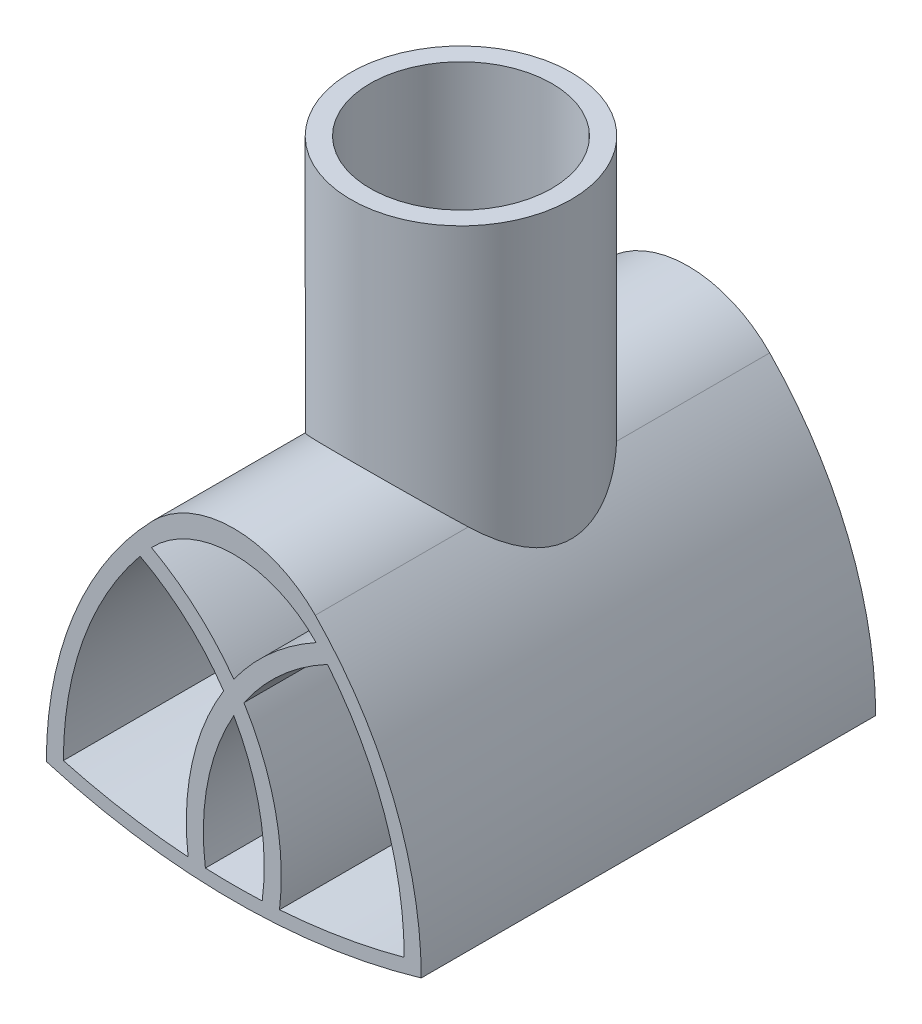
SolidWorks part; units mm, degrees
ref_plane "前视基准面" through (0, 0, 0) normal (0, 0, 1) x (1, 0, 0)
ref_plane "上视基准面" through (0, 0, 0) normal (0, 1, 0) x (1, 0, 0)
ref_plane "右视基准面" through (0, 0, 0) normal (1, 0, 0) x (0, 0, -1)
sketch "缓冲脚外形" plane through (0, 0, 0) normal (0, 0, 1) x (1, 0, 0)
  line L0 (0, 0) -> (0, -36980.811) construction
  line L1 (0, 0) -> (36980.811, 0) construction
  arc A0 (-15, 2) -> (15, 2) centre (0, 57.25) ccw
  arc A1 (-16.5, 1.1773) -> (16.5, 1.1773) centre (0, 57.25) ccw
  arc A2 (-15, 2) -> (-7.5, 21.8431) centre (15, 2) cw
  arc A3 (15, 2) -> (7.5, 21.8431) centre (-15, 2) ccw
  arc A4 (16.5, 1.1773) -> (7.1739, 24.1674) centre (-16.5, 1.1773) ccw
  arc A5 (-16.5, 1.1773) -> (-7.1739, 24.1674) centre (16.5, 1.1773) cw
  arc A6 (7.25, 22.1231) -> (-4.0228, 0.1415) centre (17.924, 2.7678) ccw
  arc A7 (-7.25, 22.1231) -> (4.0228, 0.1415) centre (-17.924, 2.7678) cw
  arc A8 (-8.25, 20.9588) -> (2.5, 0.0546) centre (-17.924, 2.7678) cw
  arc A9 (8.25, 20.9588) -> (-2.5, 0.0546) centre (17.924, 2.7678) ccw
  arc A10 (7.1739, 24.1674) -> (-7.1739, 24.1674) centre (0, 17.2007) ccw
  arc A11 (7.5, 21.8431) -> (-7.5, 21.8431) centre (0, 15.2288) ccw
  point P15 (-7.25, 22.1231)
  point P16 (7.25, 22.1231)
  point P29 (0, 29.7561)
  point P32 (0, 27.9808)
  dimension "D4" = 1.2
  dimension "D7" = 5
  dimension "D8" = 1.5
  dimension "D9" = 10
  dimension "D1" = 30
  dimension "D2" = 2
  dimension "D3" = 33
  dimension "D5" = 14.5
  dimension "D6" = 16.5
extrude "支撑脚" add sketch "缓冲脚外形" along normal mid plane 40 contours A2 A8 A6 A7 | A9 A3 A6 A7 | A7 A9 A8 A0 | A9 A7 A6 A8 | A9 A8 A6 A0 | A5 A1 A4 A3 A0 A2
ref_plane "碳管底端" through (0, 22.1207, 0) normal (0, -1, 0) x (-1, 0, 0)
sketch "碳管抱紧" plane through (0, 22.1207, 0) normal (0, -1, 0) x (-1, 0, 0)
  circle A0 centre (0, 0) radius 9.7
  circle A1 centre (0, 0) radius 8
  dimension "D1" = 16
  dimension "D2" = 19.4
extrude "连接碳管" add sketch "碳管抱紧" against normal blind 25 and the other way up to surface other way up to face at (9.5341, 0.937, 0)
sketch "镂空" plane through (0, 0, 0) normal (0, 0, 1) x (1, 0, 0)
  arc A0 (4.0228, 0.1415) -> (15, 2) centre (0, 57.25) ccw construction
  arc A1 (15, 2) -> (8.25, 20.9588) centre (-15, 2) ccw construction
  arc A2 (-8.25, 20.9588) -> (-15, 2) centre (15, 2) ccw construction
  arc A3 (-15, 2) -> (-4.0228, 0.1415) centre (0, 57.25) ccw construction
  arc A4 (-2.5, 0.0546) -> (2.5, 0.0546) centre (0, 57.25) ccw construction
  arc A5 (2.5, 0.0546) -> (0, 12.9281) centre (-17.924, 2.7678) ccw construction
  arc A6 (0, 12.9281) -> (-2.5, 0.0546) centre (17.924, 2.7678) ccw construction
  arc A7 (-0.8935, 14.3636) -> (-4.0228, 0.1415) centre (17.924, 2.7678) ccw construction
  arc A8 (-0.8935, 14.3636) -> (-8.25, 20.9588) centre (-17.924, 2.7678) ccw construction
  arc A9 (4.0228, 0.1415) -> (0.8935, 14.3636) centre (-17.924, 2.7678) ccw construction
  arc A10 (8.25, 20.9588) -> (0.8935, 14.3636) centre (17.924, 2.7678) ccw construction
  arc A11 (7.2458, 22.1207) -> (0, 15.7019) centre (17.924, 2.7678) ccw construction
  arc A12 (7.2458, 22.1207) -> (-7.2458, 22.1207) centre (0, 15.2288) ccw construction
  arc A13 (0, 15.7019) -> (-7.2458, 22.1207) centre (-17.924, 2.7678) ccw construction
  arc A14 (4.0228, 0.1415) -> (15, 2) centre (0, 57.25) ccw
  arc A15 (15, 2) -> (8.25, 20.9588) centre (-15, 2) ccw
  arc A16 (-8.25, 20.9588) -> (-15, 2) centre (15, 2) ccw
  arc A17 (-15, 2) -> (-4.0228, 0.1415) centre (0, 57.25) ccw
  arc A18 (-2.5, 0.0546) -> (2.5, 0.0546) centre (0, 57.25) ccw
  arc A19 (2.5, 0.0546) -> (0, 12.9281) centre (-17.924, 2.7678) ccw
  arc A20 (0, 12.9281) -> (-2.5, 0.0546) centre (17.924, 2.7678) ccw
  arc A21 (-0.8935, 14.3636) -> (-4.0228, 0.1415) centre (17.924, 2.7678) ccw
  arc A22 (-0.8935, 14.3636) -> (-8.25, 20.9588) centre (-17.924, 2.7678) ccw
  arc A23 (4.0228, 0.1415) -> (0.8935, 14.3636) centre (-17.924, 2.7678) ccw
  arc A24 (8.25, 20.9588) -> (0.8935, 14.3636) centre (17.924, 2.7678) ccw
  arc A25 (7.2458, 22.1207) -> (0, 15.7019) centre (17.924, 2.7678) ccw
  arc A26 (7.2458, 22.1207) -> (-7.2458, 22.1207) centre (0, 15.2288) ccw
  arc A27 (0, 15.7019) -> (-7.2458, 22.1207) centre (-17.924, 2.7678) ccw
extrude "切除-拉伸1" cut sketch "镂空" against normal through all both and the other way through all
